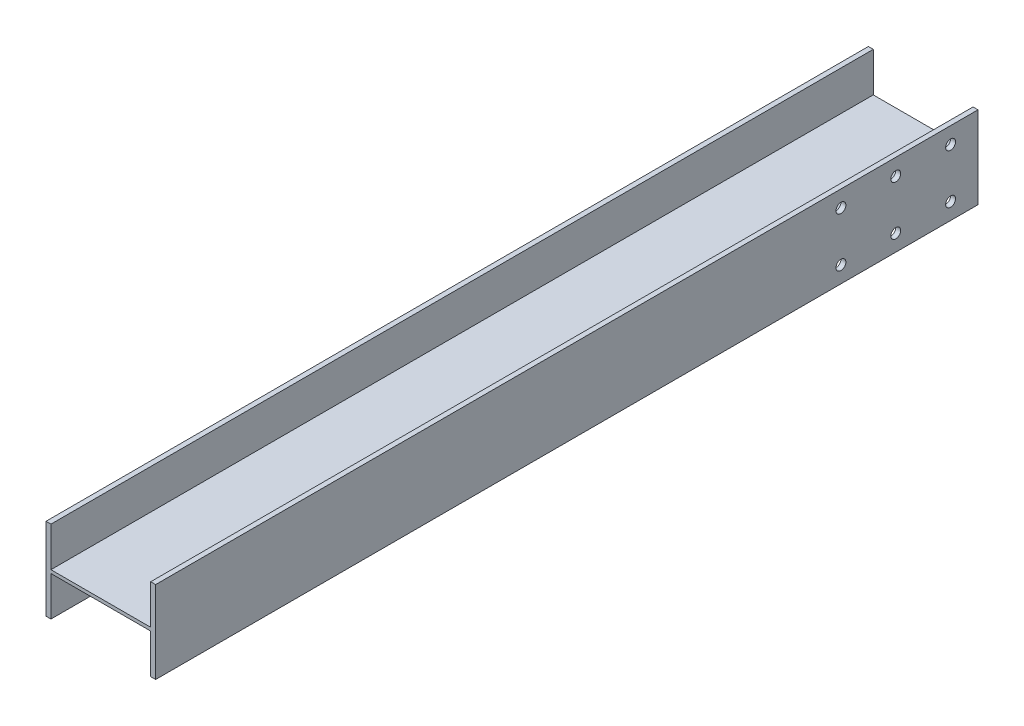
SolidWorks part; units mm, degrees
ref_plane "Front Plane" through (0, 0, 0) normal (0, 0, 1) x (1, 0, 0)
ref_plane "Top Plane" through (0, 0, 0) normal (0, 1, 0) x (1, 0, 0)
ref_plane "Right Plane" through (0, 0, 0) normal (1, 0, 0) x (0, 0, -1)
sketch "Sketch1" plane through (0, 0, 0) normal (0, 0, 1) x (1, 0, 0)
  line L0 (0, 0) -> (0, 49.8466) construction
  line L5 (97.1854, 1.5029) -> (-97, -1.5) construction
  line L6 (97, -4.5) -> (-97, 4.5) construction
  line L7 (-91, -75) -> (-100, -75)
  line L8 (-91, -75) -> (-91, -3)
  line L9 (-91, 75) -> (-100, 75)
  line L10 (-100, -75) -> (-100, 75)
  line L11 (-91, -75) -> (-100, 75) construction
  line L12 (-91, 75) -> (-100, -75) construction
  line L13 (91, -75) -> (100, -75)
  line L14 (91, 75) -> (100, -75) construction
  line L15 (91, -75) -> (100, 75) construction
  line L16 (100, -75) -> (100, 75)
  line L17 (91, 75) -> (100, 75)
  line L18 (91, -75) -> (91, -3)
  line L19 (91, 3) -> (91, 75)
  line L20 (-91, 3) -> (-91, 75)
  line L21 (91, 3) -> (-91, 3)
  line L22 (91, -3) -> (-91, -3)
  line L23 (0, 0) -> (-55.4881, 0) construction
  point P0 (0, 0)
  point P6 (-95.5, 0)
  dimension "D1" = 200
  dimension "D2" = 150
  dimension "D3" = 9
  dimension "D4" = 6
extrude "Boss-Extrude1" add sketch "Sketch1" along normal blind 1500
sketch "Sketch2" plane through (91, 0, 0) normal (-1, 0, 0) x (0, 0, 1)
  line L0 (0, 75) -> (0, -75) construction
  line L1 (1500, -75) -> (0, -75) construction
  line L2 (0, 0) -> (132.3673, 0) construction
  circle A0 centre (50, -45) radius 9
  circle A1 centre (150, -45) radius 9
  circle A2 centre (250, -45) radius 9
  circle A3 centre (250, 45) radius 9
  circle A4 centre (150, 45) radius 9
  circle A5 centre (50, 45) radius 9
  dimension "D1" = 18
  dimension "D2" = 50
  dimension "D3" = 100
  dimension "D4" = 100
  dimension "D5" = 30
extrude "Cut-Extrude1" cut sketch "Sketch2" against normal blind 1500
